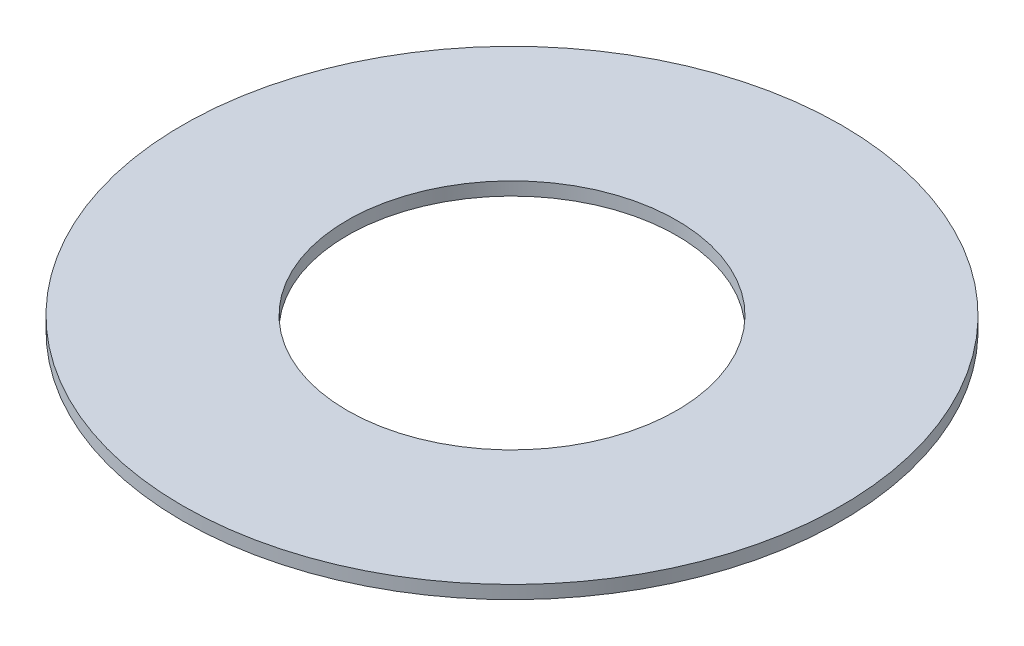
from build123d import *

# Parameters (mm, degrees)
SKETCH1_R           = 50
SKETCH1_R_2         = 25
BOSS_EXTRUDE1_DEPTH = 2


with BuildPart() as part:
    # Sketch1 → Boss-Extrude1 (new body)
    with BuildSketch(Plane(origin=(0, 0, 0), x_dir=(1, 0, 0), z_dir=(0, 1, 0))):
        with Locations(Location((0, 0, 0), (0, 0, 270))):
            Circle(SKETCH1_R)
        with Locations(Location((0, 0, 0), (0, 0, 270))):
            Circle(SKETCH1_R_2, mode=Mode.SUBTRACT)
    extrude(amount=BOSS_EXTRUDE1_DEPTH)


solid = part.part
